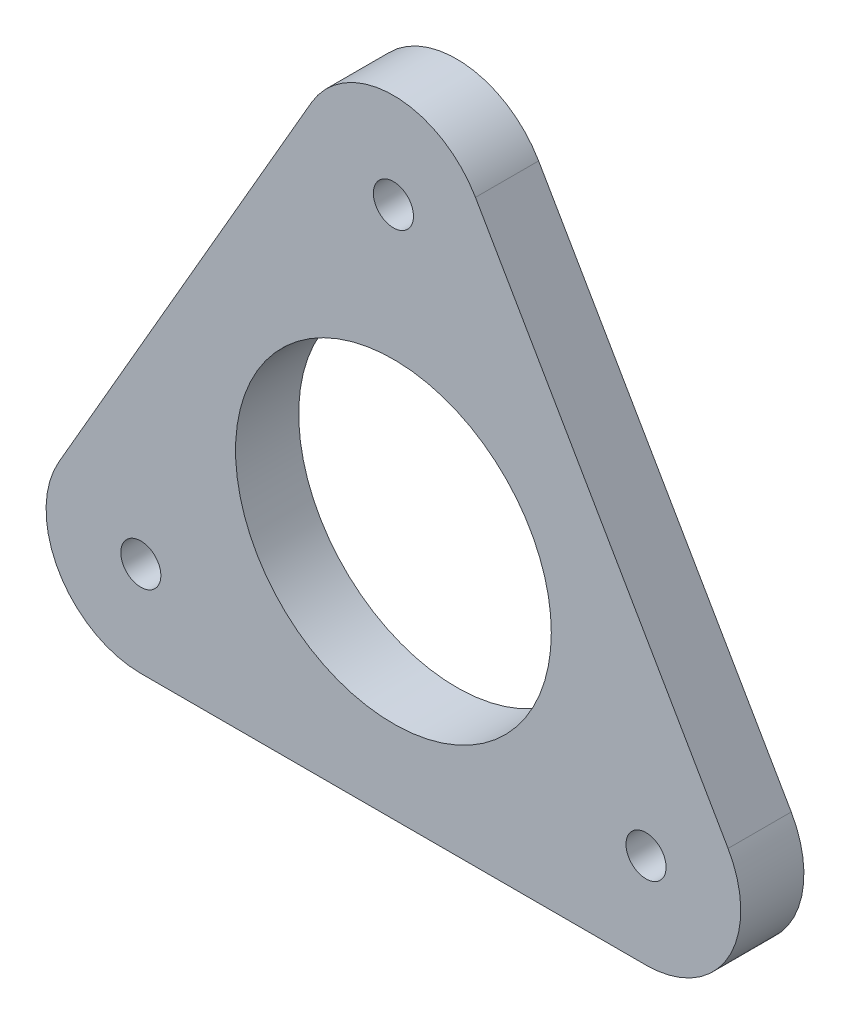
from build123d import *

# Parameters (mm, degrees)
SKETCH1_R           = 3.175
SKETCH1_R_2         = 25
BOSS_EXTRUDE1_DEPTH = 10
SKETCH2_R           = 3.175
CUT_EXTRUDE1_DEPTH  = 3
SCALE_RATIO_1_SCALE = 1.3


with BuildPart() as part:
    # Sketch1 → Boss-Extrude1 (new body)
    with BuildSketch(Plane.XY):
        with BuildLine():
            Line((-52.990381057, -15.594010768), (-12.990381057, 53.688021535))
            ThreePointArc((-12.990381057, 53.688021535), (0, 61.188021535), (12.990381057, 53.688021535))
            Line((12.990381057, 53.688021535), (52.990381057, -15.594010768))
            ThreePointArc((52.990381057, -15.594010768), (52.990381057, -30.594010768), (40, -38.094010768))
            Line((40, -38.094010768), (-40, -38.094010768))
            ThreePointArc((-40, -38.094010768), (-52.990381057, -30.594010768), (-52.990381057, -15.594010768))
        make_face()
        with Locations((-40, -23.094010768)):
            Circle(SKETCH1_R, mode=Mode.SUBTRACT)
        with Locations((40, -23.094010768)):
            Circle(SKETCH1_R, mode=Mode.SUBTRACT)
        with Locations((0, 46.188021535)):
            Circle(SKETCH1_R, mode=Mode.SUBTRACT)
        Circle(SKETCH1_R_2, mode=Mode.SUBTRACT)
    extrude(amount=BOSS_EXTRUDE1_DEPTH)

    # Sketch2 → Cut-Extrude1 (cut)
    # profile 1 of 3: a face of its own
    with BuildSketch(Plane.XY):
        with BuildLine():
            Line((-39.68174609, -27.58274271), (-46.857480139, -28.091506755))
            ThreePointArc((-46.857480139, -28.091506755), (-47.794228634, -27.594010768), (-47.75669855, -26.53401478))
            Line((-47.75669855, -26.53401478), (-43.728228938, -20.574028825))
            ThreePointArc((-43.728228938, -20.574028825), (-36.102885683, -20.844010768), (-39.68174609, -27.58274271))
        make_face()
        with Locations((-40, -23.094010768)):
            Circle(SKETCH2_R, mode=Mode.SUBTRACT)
    # profile 2 of 3: a face of its own
    with BuildSketch(Plane.XY):
        with BuildLine():
            Line((-4.046482848, 48.156771535), (-0.899218411, 54.625521535))
            ThreePointArc((-0.899218411, 54.625521535), (0, 55.188021535), (0.899218411, 54.625521535))
            Line((0.899218411, 54.625521535), (4.046482848, 48.156771535))
            ThreePointArc((4.046482848, 48.156771535), (0, 41.688021535), (-4.046482848, 48.156771535))
        make_face()
        with Locations((0, 46.188021535)):
            Circle(SKETCH2_R, mode=Mode.SUBTRACT)
    # profile 3 of 3: a face of its own
    with BuildSketch(Plane.XY):
        with BuildLine():
            Line((43.728228938, -20.574028825), (47.75669855, -26.53401478))
            ThreePointArc((47.75669855, -26.53401478), (47.794228634, -27.594010768), (46.857480139, -28.091506755))
            Line((46.857480139, -28.091506755), (39.68174609, -27.58274271))
            ThreePointArc((39.68174609, -27.58274271), (36.102885683, -20.844010768), (43.728228938, -20.574028825))
        make_face()
        with Locations((40, -23.094010768)):
            Circle(SKETCH2_R, mode=Mode.SUBTRACT)
    extrude(amount=CUT_EXTRUDE1_DEPTH, mode=Mode.SUBTRACT)


with BuildPart() as part_1:
    # Scale ratio 1: scaled about (0, 0, 0)
    add(part.part.scale(SCALE_RATIO_1_SCALE))


solid = part_1.part
